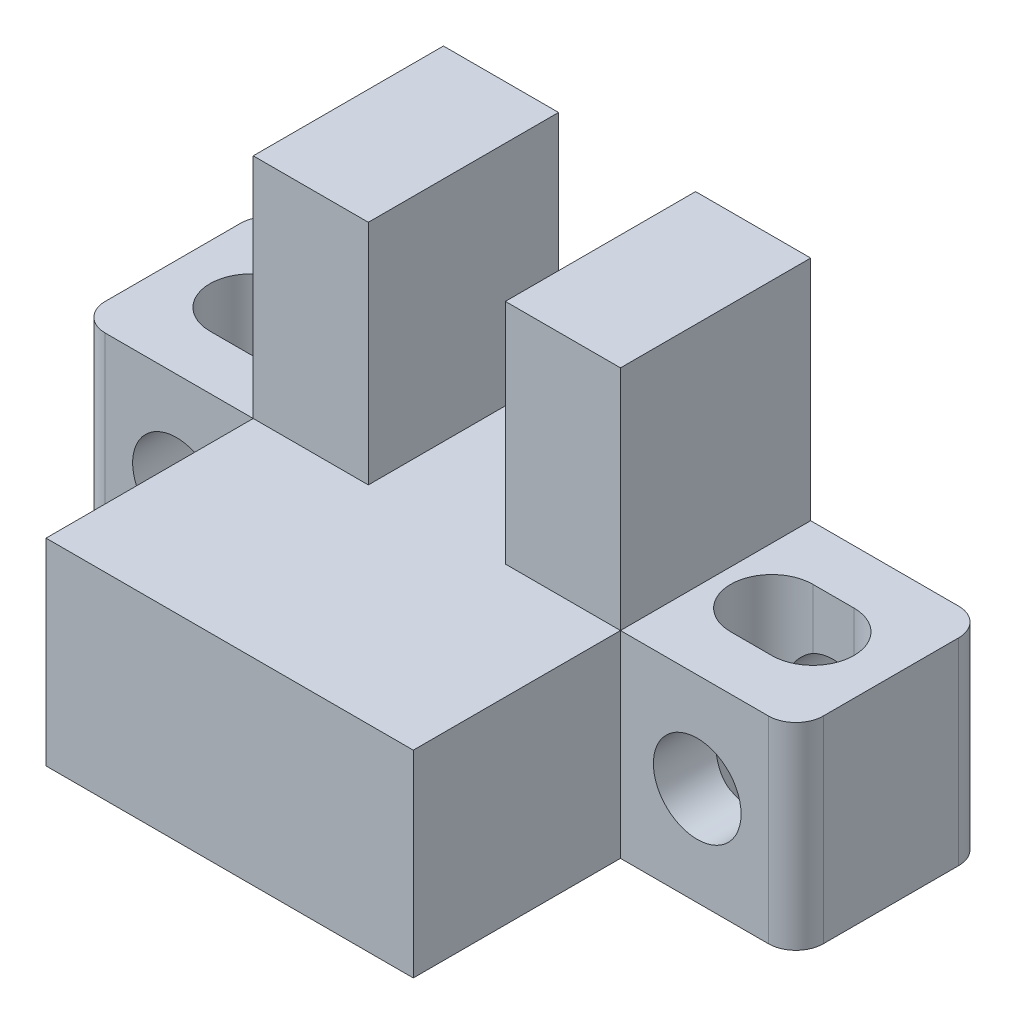
from build123d import *

# Parameters (mm, degrees)
EXTRUDE_1_DEPTH     = 7.2
SKETCH_2_W          = 4.2
SKETCH_2_H          = 6.94
EXTRUDE_2_DEPTH     = 8.3
CUT_EXTRUDE_1_DEPTH = 32.073783162
SKETCH_4_R          = 1.6
CUT_EXTRUDE_2_DEPTH = 32.366281259
FILLET_1_R          = 1


with BuildPart() as part:
    # 草图1 → 凸台-拉伸1 (new body)
    with BuildSketch(Plane(origin=(0, 0, 0), x_dir=(1, 0, 0), z_dir=(0, 1, 0))):
        Polygon((0, -6.94), (6.4, -6.94), (6.4, -14.5), (19.8, -14.5), (19.8, -6.94), (26.2, -6.94), (26.2, 0), (0, 0), align=None)
    extrude(amount=EXTRUDE_1_DEPTH)

    # 草图2 → 凸台-拉伸2 (add)
    with BuildSketch(Plane(origin=(0, 7.2, 0), x_dir=(1, 0, 0), z_dir=(0, 1, 0))):
        with Locations((8.5, -3.47)):
            Rectangle(SKETCH_2_W, SKETCH_2_H)
        with Locations((17.7, -3.47)):
            Rectangle(SKETCH_2_W, SKETCH_2_H)
    extrude(amount=EXTRUDE_2_DEPTH)

    # 草图3 → 切除-拉伸1 (cut, through all)
    with BuildSketch(Plane(origin=(0, 7.2, 0), x_dir=(1, 0, 0), z_dir=(0, 1, 0))):
        with BuildLine():
            Line((2.85, -1.97), (4.35, -1.97))
            ThreePointArc((4.35, -1.97), (5.85, -3.47), (4.35, -4.97))
            Line((4.35, -4.97), (2.85, -4.97))
            ThreePointArc((2.85, -4.97), (1.35, -3.47), (2.85, -1.97))
        make_face()
        with BuildLine():
            Line((23.35, -4.97), (21.85, -4.97))
            ThreePointArc((21.85, -4.97), (20.35, -3.47), (21.85, -1.97))
            Line((21.85, -1.97), (23.35, -1.97))
            ThreePointArc((23.35, -1.97), (24.85, -3.47), (23.35, -4.97))
        make_face()
    extrude(amount=-CUT_EXTRUDE_1_DEPTH, mode=Mode.SUBTRACT)

    # 草图4 → 切除-拉伸2 (cut, through all)
    with BuildSketch(Plane.XY.offset(6.94)):
        with Locations((22.6, 3.6)):
            Circle(SKETCH_4_R)
        with Locations((3.6, 3.6)):
            Circle(SKETCH_4_R)
    extrude(amount=-CUT_EXTRUDE_2_DEPTH, mode=Mode.SUBTRACT)

    # 圆角1
    fillet_1_edges = [part.edges().sort_by_distance(p)[0] for p in [
        (0, 3.6, 0),
        (0, 3.6, 6.94),
        (26.2, 3.6, 0),
        (26.2, 3.6, 6.94),
    ]]
    fillet(fillet_1_edges, radius=FILLET_1_R)


solid = part.part
